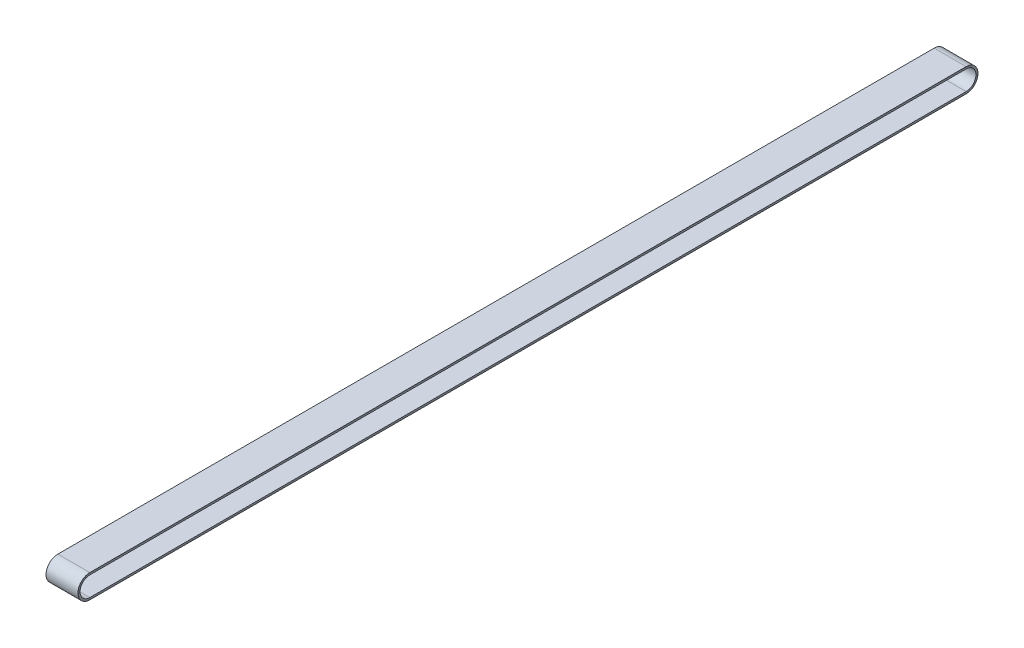
SolidWorks part; units mm, degrees
ref_plane "前基準面" through (0, 0, 0) normal (0, 0, 1) x (1, 0, 0)
ref_plane "上基準面" through (0, 0, 0) normal (0, 1, 0) x (1, 0, 0)
ref_plane "右基準面" through (0, 0, 0) normal (1, 0, 0) x (0, 0, -1)
sketch "草图1" plane through (0, 0, 0) normal (1, 0, 0) x (0, 0, -1)
  line L0 (0, 0) -> (2192.5, 0) construction
  line L1 (0, 27.325) -> (2192.5, 27.325)
  line L2 (0, -27.325) -> (2192.5, -27.325)
  arc A1 (0, 27.325) -> (0, -27.325) centre (0, 0) ccw
  arc A2 (2192.5, -27.325) -> (2192.5, 27.325) centre (2192.5, 0) ccw
  point P3 (1096.25, 0)
  dimension "D1" = 54.65
  dimension "D2" = 2192.5
extrude "拉伸-薄壁1" add sketch "草图1" along normal mid plane 80 thin thin type one direction wall 2.25
sketch "草图2" plane through (0, 0, 0) normal (1, 0, 0) x (0, 0, -1)
  line L2 (2192.5, 27.325) -> (0, 27.325)
  line L3 (0, -27.325) -> (2192.5, -27.325)
  line L4 (2192.5, 27.325) -> (0, 27.325)
  line L5 (0, -27.325) -> (2192.5, -27.325)
  arc A2 (2192.5, -27.325) -> (2192.5, 27.325) centre (2192.5, 0) ccw
  arc A3 (0, 27.325) -> (0, -27.325) centre (0, 0) ccw
  arc A4 (2192.5, -27.325) -> (2192.5, 27.325) centre (2192.5, 0) ccw
  arc A5 (0, 27.325) -> (0, -27.325) centre (0, 0) ccw
  dimension "D1" = 0
extrude "拉伸-薄壁2" add sketch "草图2" along normal mid plane 80 separate body thin thin type one direction reverse wall 2.83
